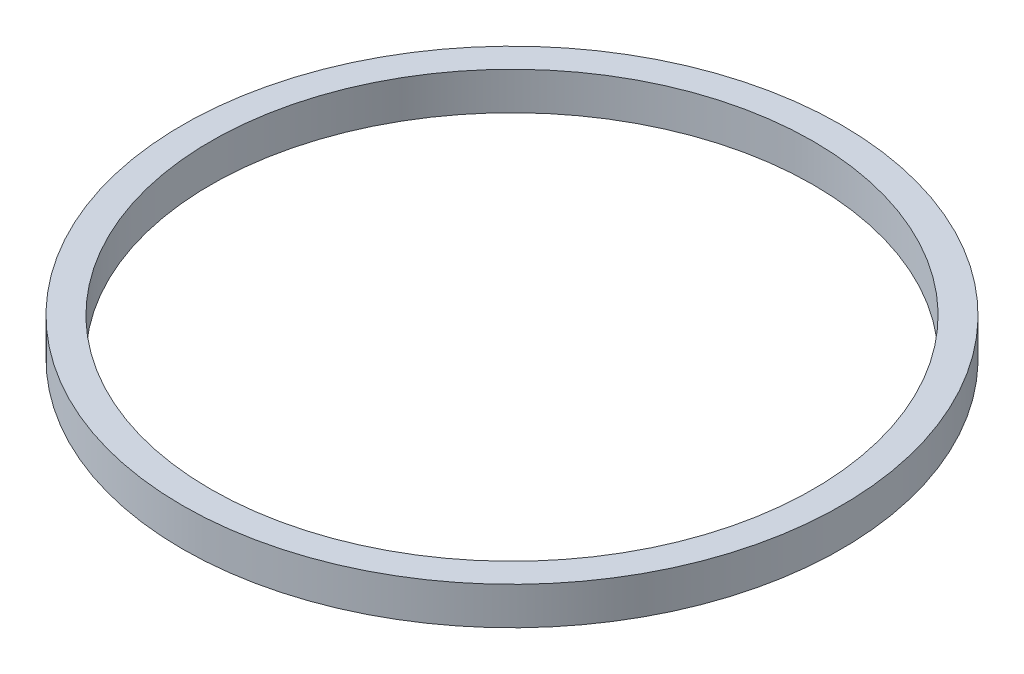
from build123d import *

# Parameters (mm, degrees)
SKETCH1_R           = 17.5
SKETCH1_R_2         = 16
BOSS_EXTRUDE1_DEPTH = 1


with BuildPart() as part:
    # Sketch1 → Boss-Extrude1 (new, symmetric)
    with BuildSketch(Plane(origin=(0, 0, 0), x_dir=(1, 0, 0), z_dir=(0, 1, 0))):
        with Locations(Location((0, 0, 0), (0, 0, 270))):
            Circle(SKETCH1_R)
        with Locations(Location((0, 0, 0), (0, 0, 270))):
            Circle(SKETCH1_R_2, mode=Mode.SUBTRACT)
    extrude(amount=BOSS_EXTRUDE1_DEPTH, both=True)


solid = part.part
